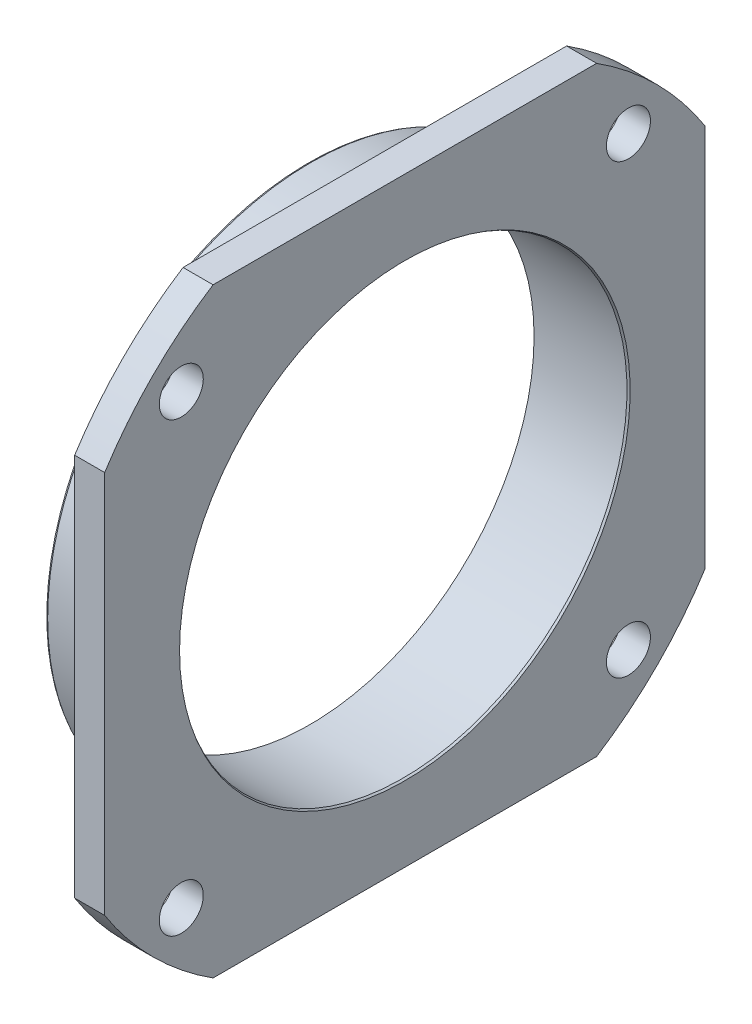
from build123d import *

# Parameters (mm, degrees)
SKETCH2_R          = 11
CUT_EXTRUDE1_DEPTH = 15
CIRPATTERN1_COUNT  = 4
CUT_EXTRUDE2_DEPTH = 15
CHAMFER1_SIZE      = 1
CHAMFER1_SIZE2     = 0.577350269
CHAMFER2_SIZE      = 1
CHAMFER2_SIZE2     = 0.577350269
CHAMFER3_SIZE      = 1
CHAMFER3_SIZE2     = 0.577350269


with BuildPart() as part:
    # Sketch1 → Revolve1 (revolve)
    with BuildSketch(Plane.XY, mode=Mode.PRIVATE) as revolve1_sk:
        Polygon((-36.947368421, 131.5), (-3.947368421, 131.5), (-3.947368421, 178), (11.052631579, 178), (11.052631579, 112), (-36.947368421, 112), align=None)
    revolve(revolve1_sk.sketch.rotate(Axis((-77.413533835, 0, 0), (1, 0, 0)), 90), axis=Axis((-77.413533835, 0, 0), (1, 0, 0)))

    # Sketch2 → Cut-Extrude1 (cut)
    with BuildSketch(Plane(origin=(11.052631579, 0, 0), x_dir=(0, 0, -1), z_dir=(1, 0, 0))):
        with Locations((111.722871427, 111.722871427)):
            Circle(SKETCH2_R)
    cut_extrude1 = extrude(amount=-CUT_EXTRUDE1_DEPTH, mode=Mode.SUBTRACT)

    # CirPattern1: Cut-Extrude1 ×4 about axis
    cirpattern1_axis = Axis((0, 0, 0), (1, 0, 0))
    for i in range(1, CIRPATTERN1_COUNT):
        add(cut_extrude1.rotate(cirpattern1_axis, i * 360 / CIRPATTERN1_COUNT), mode=Mode.SUBTRACT)

    # Sketch3 → Cut-Extrude2 (cut)
    with BuildSketch(Plane(origin=(11.052631579, 0, 0), x_dir=(0, 0, -1), z_dir=(1, 0, 0))):
        with BuildLine():
            Line((-95.833188406, 150), (95.833188406, 150))
            ThreePointArc((95.833188406, 150), (0, 178), (-95.833188406, 150))
        make_face()
        with BuildLine():
            Line((-150, 95.833188406), (-150, -95.833188406))
            ThreePointArc((-150, -95.833188406), (-178, 0), (-150, 95.833188406))
        make_face()
        with BuildLine():
            Line((-95.833188406, -150), (95.833188406, -150))
            ThreePointArc((95.833188406, -150), (0, -178), (-95.833188406, -150))
        make_face()
        with BuildLine():
            Line((150, 95.833188406), (150, -95.833188406))
            ThreePointArc((150, -95.833188406), (178, 0), (150, 95.833188406))
        make_face()
    extrude(amount=-CUT_EXTRUDE2_DEPTH, mode=Mode.SUBTRACT)

    # Chamfer1
    chamfer1_edges = [part.edges().sort_by_distance(p)[0] for p in [
        (11.052631579, 0, -112),
    ]]
    chamfer1_side = [part.faces().sort_by_distance(p)[0] for p in [
        (-12.947368421, 0, -112),
    ]]
    chamfer(chamfer1_edges, length=CHAMFER1_SIZE, length2=CHAMFER1_SIZE2, reference=chamfer1_side[0])

    # Chamfer2
    chamfer2_edges = [part.edges().sort_by_distance(p)[0] for p in [
        (-36.947368421, 0, -112),
    ]]
    chamfer2_side = [part.faces().sort_by_distance(p)[0] for p in [
        (-36.947368421, 0, -115.719381669),
    ]]
    chamfer(chamfer2_edges, length=CHAMFER2_SIZE, length2=CHAMFER2_SIZE2, reference=chamfer2_side[0])

    # Chamfer3
    chamfer3_edges = [part.edges().sort_by_distance(p)[0] for p in [
        (-36.947368421, 0, -131.5),
    ]]
    chamfer3_side = [part.faces().sort_by_distance(p)[0] for p in [
        (-20.447368421, 0, -131.5),
    ]]
    chamfer(chamfer3_edges, length=CHAMFER3_SIZE, length2=CHAMFER3_SIZE2, reference=chamfer3_side[0])


solid = part.part
